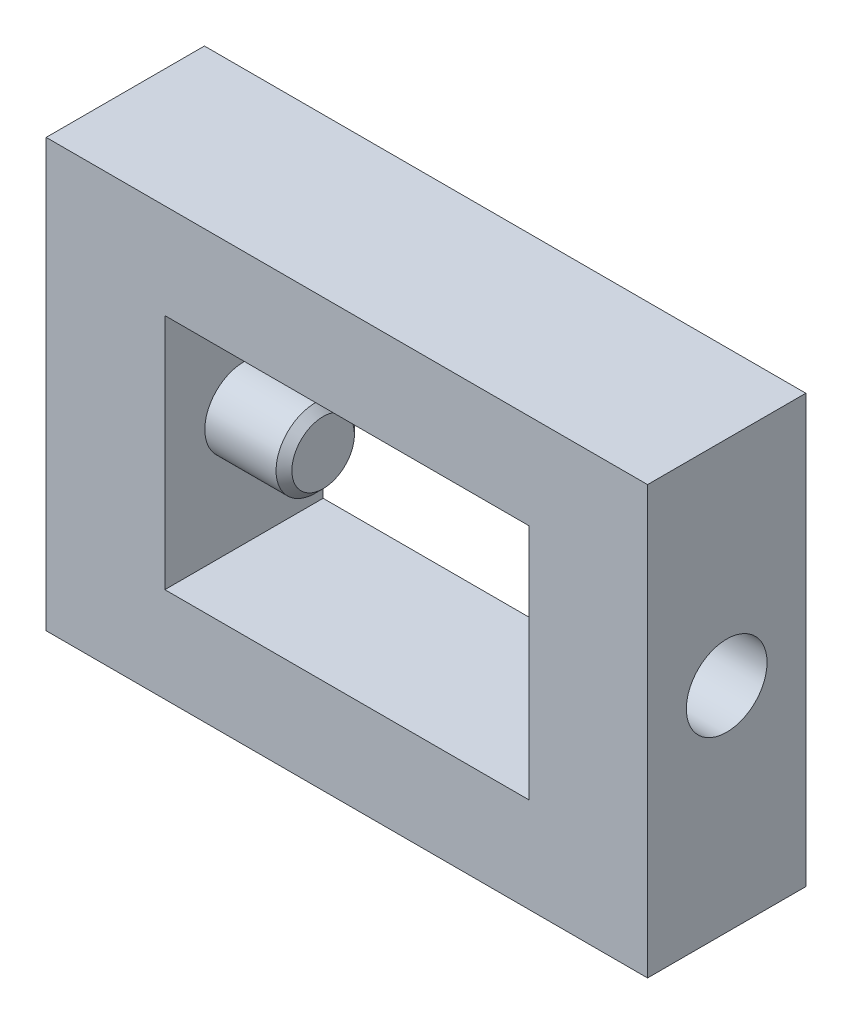
from build123d import *

# Parameters (mm, degrees)
SKETCH_1_W              = 76
SKETCH_1_H              = 54
SKETCH_1_W_2            = 46
SKETCH_1_H_2            = 30
EXTRUDE_1_DEPTH         = 10
SKETCH_2_R              = 4.95
CUT_EXTRUDE_1_DEPTH     = 20
HOLE_WIZARD_M12_1_D     = 10.2
HOLE_WIZARD_M12_1_DEPTH = 32.75
HOLE_WIZARD_M12_1_TIP   = 3.064389157
SKETCH_5_R              = 4.95
EXTRUDE_2_DEPTH         = 25
CHAMFER_1_SIZE          = 1


with BuildPart() as part:
    # 草图1 → 凸台-拉伸1 (new, symmetric)
    with BuildSketch(Plane.XY):
        Rectangle(SKETCH_1_W, SKETCH_1_H)
        Rectangle(SKETCH_1_W_2, SKETCH_1_H_2, mode=Mode.SUBTRACT)
    extrude(amount=EXTRUDE_1_DEPTH, both=True)

    # 草图2 → 切除-拉伸1 (cut)
    with BuildSketch(Plane.ZY.offset(38)):
        with Locations(Location((0, 0, 0), (0, 0, 270))):
            Circle(SKETCH_2_R)
    extrude(amount=-CUT_EXTRUDE_1_DEPTH, mode=Mode.SUBTRACT)

    # M12 螺纹孔1
    with Locations(Plane(origin=(38, 0, 0), x_dir=(0, 0, -1), z_dir=(1, 0, 0))):
        with Locations((0, 0)):
            Hole(HOLE_WIZARD_M12_1_D / 2, depth=HOLE_WIZARD_M12_1_DEPTH)
            with Locations((0, 0, -(HOLE_WIZARD_M12_1_DEPTH + HOLE_WIZARD_M12_1_TIP / 2))):  # 118° drill point
                Cone(0, HOLE_WIZARD_M12_1_D / 2, HOLE_WIZARD_M12_1_TIP, mode=Mode.SUBTRACT)


with BuildPart() as body_2:
    # 草图5 → 凸台-拉伸2 (new body)
    with BuildSketch(Plane.ZY.offset(38)):
        with Locations(Location((0, 0, 0), (0, 0, 270))):
            Circle(SKETCH_5_R)
    extrude(amount=-EXTRUDE_2_DEPTH)

    # 倒角1
    chamfer_1_edges = [body_2.edges().sort_by_distance(p)[0] for p in [
        (-38, 4.95, 0),
        (-13, 4.95, 0),
    ]]
    chamfer(chamfer_1_edges, length=CHAMFER_1_SIZE)


solid = Compound([part.part, body_2.part])
